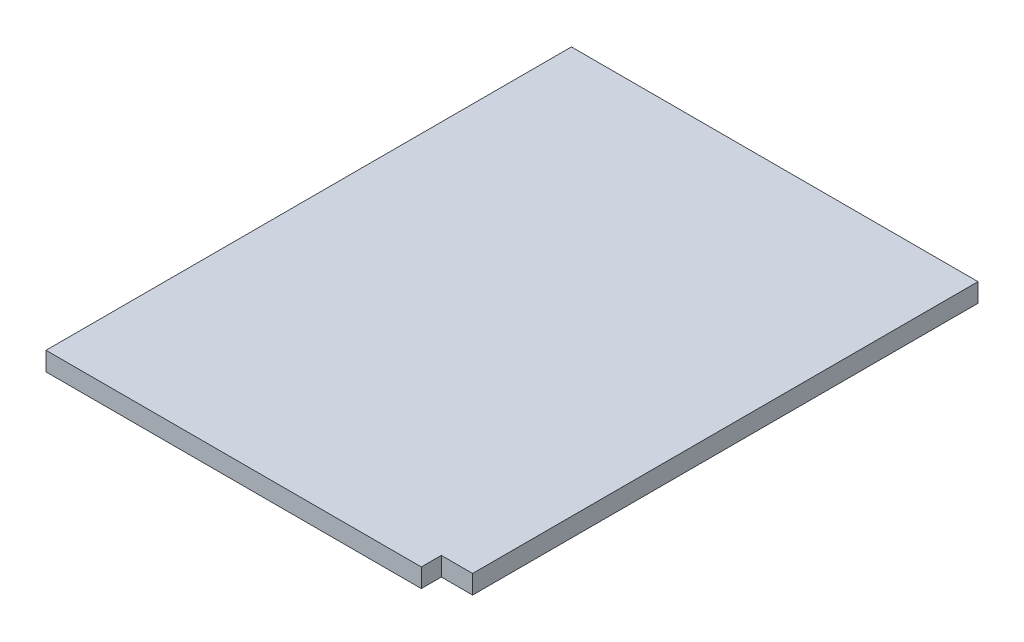
from build123d import *

# Parameters (mm, degrees)
BOSS_EXTRUDE1_DEPTH = 15


with BuildPart() as part:
    # Sketch1 → Boss-Extrude1 (new body)
    with BuildSketch(Plane.XZ):
        Polygon((300, 420), (0, 420), (0, 0), (325, 0), (325, 404), (300, 404), align=None)
    extrude(amount=-BOSS_EXTRUDE1_DEPTH)


solid = part.part
